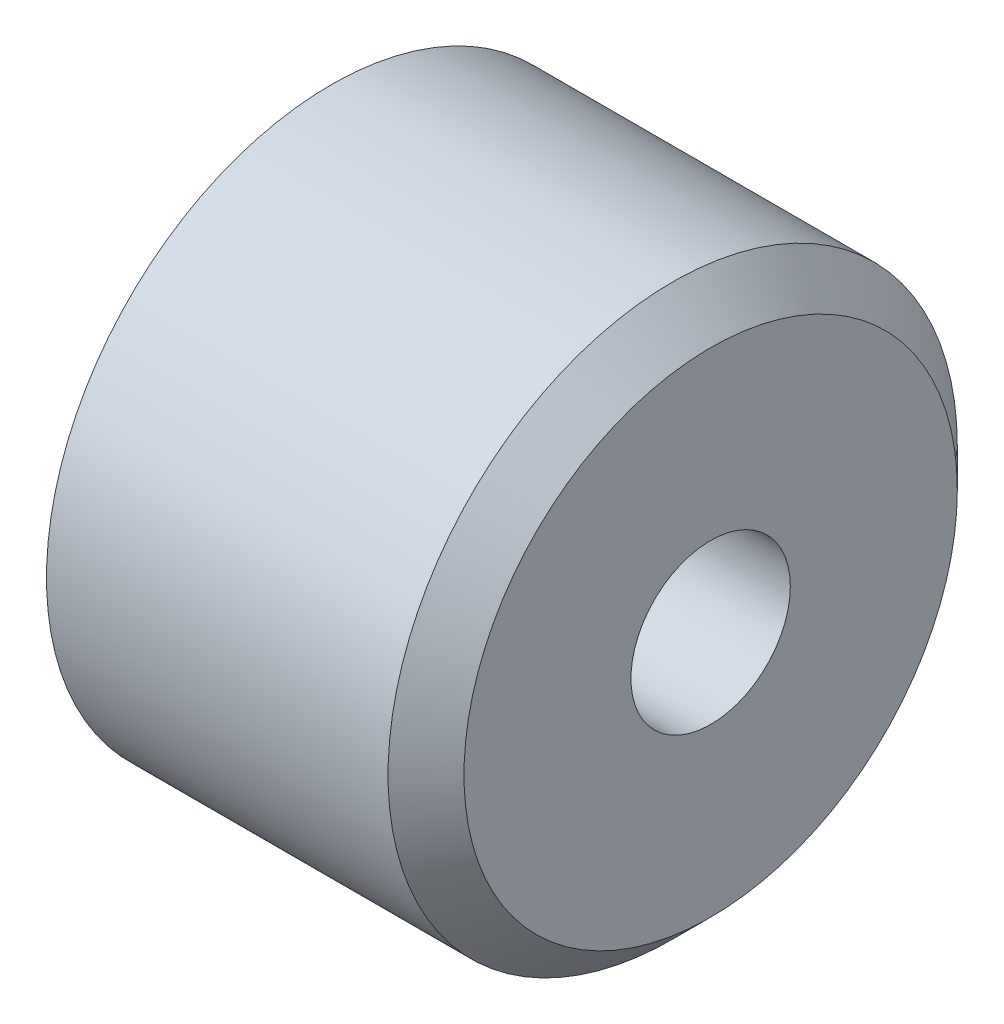
SolidWorks part; units mm, degrees
material "1023 碳钢板 (SS)"
ref_plane "Front Plane" through (0, 0, 0) normal (0, 0, 1) x (1, 0, 0)
ref_plane "Top Plane" through (0, 0, 0) normal (0, 1, 0) x (1, 0, 0)
ref_plane "Right Plane" through (0, 0, 0) normal (1, 0, 0) x (0, 0, -1)
sketch "Sketch1" plane through (2.5, 0, 0) normal (1, 0, 0) x (0, 0, -1)
  circle A0 centre (-39.5, 200) radius 7.5
extrude "Boss-Extrude1" add sketch "Sketch1" along normal blind 10
chamfer "Chamfer1" distance 1 angle 45 1 edges at (12.5, 200, 32)
hole_wizard "M5 Tapped Hole1" positions "3DSketch2" profile "Sketch3" tap size "M5" standard "IS"
sketch3d "3DSketch2"
  line L0 (11.5, 200, 39.5) -> (12.5, 200, 39.5) construction
  point P0 (12.5, 200, 39.5)
sketch "Sketch3" plane through (12.5, 200, 39.5) normal (0, 1, 0) x (0, 0, -1)
  line L0 (0, 0) -> (0, 11.2618)
  line L1 (0, 11.2618) -> (2.1, 10)
  line L2 (2.1, 10) -> (2.1, 0)
  line L5 (2.1, 0) -> (0, 0)
  line L10 (0, 11.2618) -> (-2.1, 10) construction
  line L11 (0, -6.35) -> (0, 107.95) construction
  dimension "螺纹孔钻头直径" = 4.2
  dimension "螺纹孔钻头深度" = 10
  dimension "导头角度" = 118
cosmetic thread "Cosmetic thread 1" parameters "D1"=10, "D2"=5
